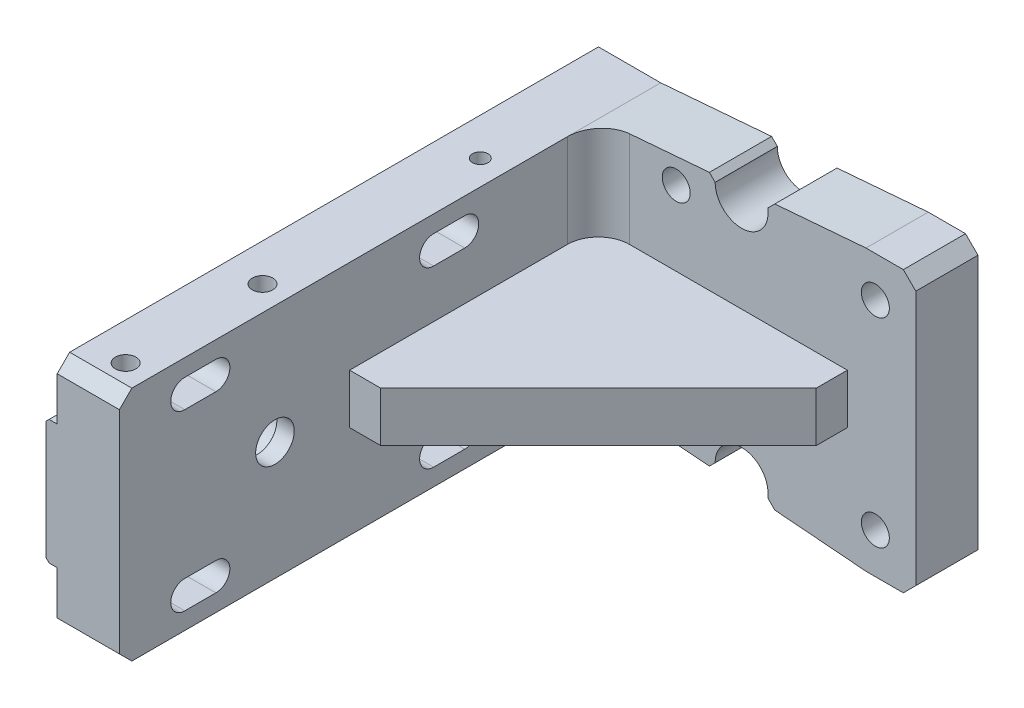
from build123d import *
from OCP.BRepFilletAPI import BRepFilletAPI_MakeChamfer

# Parameters (mm, degrees)
SKETCH1_W             = 61
SKETCH1_H             = 45
BOSS_EXTRUDE1_DEPTH   = 10
SKETCH2_W             = 10
SKETCH2_H             = 45
BOSS_EXTRUDE2_DEPTH   = 77
CUT_EXTRUDE3_DEPTH    = 104.325940596
SKETCH6_W             = 40
SKETCH6_H             = 8
BOSS_EXTRUDE3_DEPTH   = 40
CUT_EXTRUDE4_DEPTH    = 96.924449438
FILLET1_R             = 5
CUT_EXTRUDE5_DEPTH    = 95.897312923
LPATTERN2_COUNT       = 2
LPATTERN2_PITCH       = 28
LPATTERN2_COUNT_DIR2  = 2
LPATTERN2_PITCH_DIR2  = 40
SKETCH9_R             = 3
CUT_EXTRUDE6_DEPTH    = 5
SKETCH10_R            = 2.25
CUT_EXTRUDE7_DEPTH    = 95.897312923
CHAMFER1_SIZE         = 2
M4_TAPPED_HOLE1_D     = 3.3
M4_TAPPED_HOLE1_DEPTH = 10.1
M4_TAPPED_HOLE1_TIP   = 0.991420021
SKETCH4_W             = 87
SKETCH4_H             = 20
BOSS_EXTRUDE4_DEPTH   = 1.8
CHAMFER2_SIZE         = 0.5
SKETCH15_R            = 3.1
CUT_EXTRUDE8_DEPTH    = 104.325940596
SKETCH16_R            = 4.05
CUT_EXTRUDE9_DEPTH    = 9
CUT_EXTRUDE10_DEPTH   = 87.478552254
CHAMFER3_SIZE         = 1
CHAMFER3_SIZE2        = 0.927789392
CHAMFER3_SIZE2_2      = 1.092207765


with BuildPart() as part:
    # Sketch1 → Boss-Extrude1 (new body)
    with BuildSketch(Plane.XY):
        Rectangle(SKETCH1_W, SKETCH1_H)
    extrude(amount=BOSS_EXTRUDE1_DEPTH)

    # Sketch2 → Boss-Extrude2 (add)
    with BuildSketch(Plane.XY.offset(10)):
        with Locations((-25.5, 0)):
            Rectangle(SKETCH2_W, SKETCH2_H)
    extrude(amount=BOSS_EXTRUDE2_DEPTH)

    # Sketch5 → Cut-Extrude3 (cut, through all)
    with BuildSketch(Plane(origin=(-20.5, 0, 0), x_dir=(0, 0, -1), z_dir=(1, 0, 0))):
        with BuildLine():
            Line((-76.5, -11.75), (-71.5, -11.75))
            ThreePointArc((-71.5, -11.75), (-69.25, -14), (-71.5, -16.25))
            Line((-71.5, -16.25), (-76.5, -16.25))
            ThreePointArc((-76.5, -16.25), (-78.75, -14), (-76.5, -11.75))
        make_face()
    cut_extrude3 = extrude(amount=-CUT_EXTRUDE3_DEPTH, mode=Mode.SUBTRACT)

    # Sketch6 → Boss-Extrude3 (add)
    with BuildSketch(Plane.XY.offset(10)):
        with Locations((-0.5, 0)):
            Rectangle(SKETCH6_W, SKETCH6_H)
    extrude(amount=BOSS_EXTRUDE3_DEPTH)

    # Sketch7 → Cut-Extrude4 (cut, through all)
    with BuildSketch(Plane.XZ.offset(4)):
        Polygon((19.5, 50), (-15.5, 50), (19.5, 15), align=None)
    extrude(amount=-CUT_EXTRUDE4_DEPTH, mode=Mode.SUBTRACT)

    # Fillet1
    fillet1_edges = [part.edges().sort_by_distance(p)[0] for p in [
        (-20.5, 13.25, 10),
        (-20.5, -13.25, 10),
    ]]
    fillet(fillet1_edges, radius=FILLET1_R)

    # Sketch8 → Cut-Extrude5 (cut, through all)
    with BuildSketch(Plane.XY.offset(87)):
        Polygon((-30.5, 22.5), (22.5, 22.5), (-20.5, 19), (-30.5, 19), align=None)
        Polygon((-20.5, -19), (22.5, -22.5), (-30.5, -22.5), (-30.5, -19), align=None)
    extrude(amount=-CUT_EXTRUDE5_DEPTH, mode=Mode.SUBTRACT)

    # LPattern2: Cut-Extrude3 2 × 2
    with Locations(*[(0, i * LPATTERN2_PITCH, -j * LPATTERN2_PITCH_DIR2) for i in range(LPATTERN2_COUNT) for j in range(LPATTERN2_COUNT_DIR2) if (i, j) != (0, 0)]):
        add(cut_extrude3, mode=Mode.SUBTRACT)

    # Sketch9 → Cut-Extrude6 (cut)
    with BuildSketch(Plane(origin=(0, 0, 0), x_dir=(-1, 0, 0), z_dir=(0, 0, -1))):
        with Locations((-25, 0)):
            Circle(SKETCH9_R)
        with BuildLine():
            Line((8.75, -3), (7.25, -3))
            ThreePointArc((7.25, -3), (4.25, 0), (7.25, 3))
            Line((7.25, 3), (8.75, 3))
            ThreePointArc((8.75, 3), (11.75, 0), (8.75, -3))
        make_face()
    extrude(amount=-CUT_EXTRUDE6_DEPTH, mode=Mode.SUBTRACT)

    # Sketch10 → Cut-Extrude7 (cut, through all)
    with BuildSketch(Plane(origin=(0, 0, 0), x_dir=(-1, 0, 0), z_dir=(0, 0, -1))):
        with Locations((8, -16)):
            Circle(SKETCH10_R)
        with Locations((-24, -16)):
            Circle(SKETCH10_R)
        with Locations((-24, 16)):
            Circle(SKETCH10_R)
        with Locations((8, 16)):
            Circle(SKETCH10_R)
    extrude(amount=-CUT_EXTRUDE7_DEPTH, mode=Mode.SUBTRACT)

    # Chamfer1
    chamfer1_edges = [part.edges().sort_by_distance(p)[0] for p in [
        (30.5, -22.5, 5),
        (30.5, 22.5, 5),
        (-25.5, -19, 87),
        (-25.5, 19, 87),
    ]]
    chamfer(chamfer1_edges, length=CHAMFER1_SIZE)

    # M4 Tapped Hole1
    with Locations(Plane(origin=(0, 19, 0), x_dir=(1, 0, 0), z_dir=(0, 1, 0))):
        with Locations((-24.5, -82), (-24.5, -60)):
            Hole(M4_TAPPED_HOLE1_D / 2, depth=M4_TAPPED_HOLE1_DEPTH)
            with Locations((0, 0, -(M4_TAPPED_HOLE1_DEPTH + M4_TAPPED_HOLE1_TIP / 2))):  # 118° drill point
                Cone(0, M4_TAPPED_HOLE1_D / 2, M4_TAPPED_HOLE1_TIP, mode=Mode.SUBTRACT)

    # Sketch13 → M3 Tapped Hole1 (revolve, cut)
    with BuildSketch(Plane(origin=(-24.5, 19, 25), x_dir=(0, 0, 1), z_dir=(1, 0, 0))):
        Polygon((0, 0), (0, 8.251075774), (1.25, 7.5), (1.25, 0), align=None)
    m3_tapped_hole1 = revolve(axis=Axis((-24.5, 25.35, 25), (0, -1, 0)), mode=Mode.SUBTRACT)

    # Mirror1: M3 Tapped Hole1 across plane
    add(m3_tapped_hole1.mirror(Plane.ZX), mode=Mode.SUBTRACT)

    # Sketch4 → Boss-Extrude4 (add)
    with BuildSketch(Plane.ZY.offset(30.5)):
        with Locations((43.5, 0)):
            Rectangle(SKETCH4_W, SKETCH4_H)
    extrude(amount=BOSS_EXTRUDE4_DEPTH)

    # Chamfer2
    chamfer2_edges = [part.edges().sort_by_distance(p)[0] for p in [
        (-32.3, 10, 43.5),
        (-32.3, -10, 43.5),
    ]]
    chamfer(chamfer2_edges, length=CHAMFER2_SIZE)

    # Sketch15 → Cut-Extrude8 (cut, through all)
    with BuildSketch(Plane(origin=(-20.5, 0, 0), x_dir=(0, 0, -1), z_dir=(1, 0, 0))):
        with Locations(Location((-62, 0, 0), (0, 0, 90))):
            Circle(SKETCH15_R)
    extrude(amount=-CUT_EXTRUDE8_DEPTH, mode=Mode.SUBTRACT)

    # Sketch16 → Cut-Extrude9 (cut)
    with BuildSketch(Plane.ZY.offset(32.3)):
        with Locations((62, 0)):
            Circle(SKETCH16_R)
    extrude(amount=-CUT_EXTRUDE9_DEPTH, mode=Mode.SUBTRACT)

    # Sketch17 → Cut-Extrude10 (cut, through all)
    with BuildSketch(Plane.XY.offset(10)):
        with BuildLine():
            Line((6.75, -19.5), (6.75, -25.912135635))
            ThreePointArc((6.75, -25.912135635), (2.5, -30.162135635), (-1.75, -25.912135635))
            Line((-1.75, -25.912135635), (-1.75, -19.5))
            ThreePointArc((-1.75, -19.5), (2.5, -15.25), (6.75, -19.5))
        make_face()
        with BuildLine():
            Line((-1.75, 19.5), (-1.75, 25.912135635))
            ThreePointArc((-1.75, 25.912135635), (2.5, 30.162135635), (6.75, 25.912135635))
            Line((6.75, 25.912135635), (6.75, 19.5))
            ThreePointArc((6.75, 19.5), (2.5, 15.25), (-1.75, 19.5))
        make_face()
    extrude(amount=-CUT_EXTRUDE10_DEPTH, mode=Mode.SUBTRACT)

    # Chamfer3: one chamfer whose edges measure the first distance from different faces: ONE call of the kernel's chamfer builder (chamfer() names one face for all edges)
    chamfer3_edges_1 = [part.edges().sort_by_distance(p)[0] for p in [
        (-1.75, -20.526162791, 5),
    ]]
    chamfer3_side_1 = [part.faces().sort_by_distance(p)[0] for p in [
        (-1.75, -20.013081395, 5),
    ]]
    chamfer3_edges_2 = [part.edges().sort_by_distance(p)[0] for p in [
        (6.75, -21.218023256, 5),
    ]]
    chamfer3_side_2 = [part.faces().sort_by_distance(p)[0] for p in [
        (6.75, -20.359011628, 5),
    ]]
    chamfer3_edges_3 = [part.edges().sort_by_distance(p)[0] for p in [
        (6.75, 21.218023256, 5),
    ]]
    chamfer3_side_3 = [part.faces().sort_by_distance(p)[0] for p in [
        (6.75, 20.359011628, 5),
    ]]
    chamfer3_edges_4 = [part.edges().sort_by_distance(p)[0] for p in [
        (-1.75, 20.526162791, 5),
    ]]
    chamfer3_side_4 = [part.faces().sort_by_distance(p)[0] for p in [
        (-1.75, 20.013081395, 5),
    ]]
    chamfer3 = BRepFilletAPI_MakeChamfer(part.part.solid().wrapped)
    for e in chamfer3_edges_1:
        chamfer3.Add(CHAMFER3_SIZE, CHAMFER3_SIZE2, e.wrapped, chamfer3_side_1[0].wrapped)  # the first distance lies on this face
    for e in chamfer3_edges_2:
        chamfer3.Add(CHAMFER3_SIZE, CHAMFER3_SIZE2_2, e.wrapped, chamfer3_side_2[0].wrapped)  # the first distance lies on this face
    for e in chamfer3_edges_3:
        chamfer3.Add(CHAMFER3_SIZE, CHAMFER3_SIZE2_2, e.wrapped, chamfer3_side_3[0].wrapped)  # the first distance lies on this face
    for e in chamfer3_edges_4:
        chamfer3.Add(CHAMFER3_SIZE, CHAMFER3_SIZE2, e.wrapped, chamfer3_side_4[0].wrapped)  # the first distance lies on this face
    add(Compound.cast(chamfer3.Shape()), mode=Mode.REPLACE)


solid = part.part
